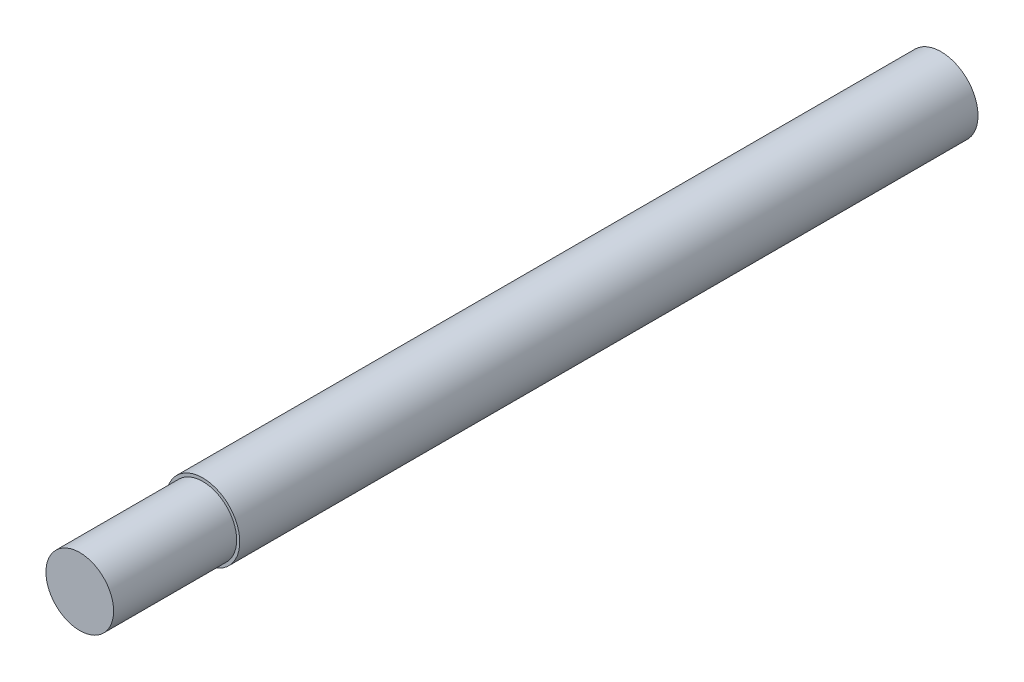
SolidWorks part; units mm, degrees
ref_plane "前视基准面" through (0, 0, 0) normal (0, 0, 1) x (1, 0, 0)
ref_plane "上视基准面" through (0, 0, 0) normal (0, 1, 0) x (1, 0, 0)
ref_plane "右视基准面" through (0, 0, 0) normal (1, 0, 0) x (0, 0, -1)
sketch "草图1" plane through (0, 0, 0) normal (0, 0, 1) x (1, 0, 0)
  circle A0 centre (0, 0) radius 6
  dimension "D1" = 12
extrude "凸台-拉伸3" add sketch "草图1" along normal mid plane 140
sketch "草图3" plane through (0, 0, 70) normal (0, 0, 1) x (1, 0, 0)
  circle A0 centre (0, 0) radius 5.5
  circle A1 centre (0, 0) radius 6 construction
  circle A2 centre (0, 0) radius 6
  dimension "D1" = 11
extrude "切除-拉伸1" cut sketch "草图3" against normal blind 20
cosmetic thread "装饰螺纹线1" parameters "D2"=10
